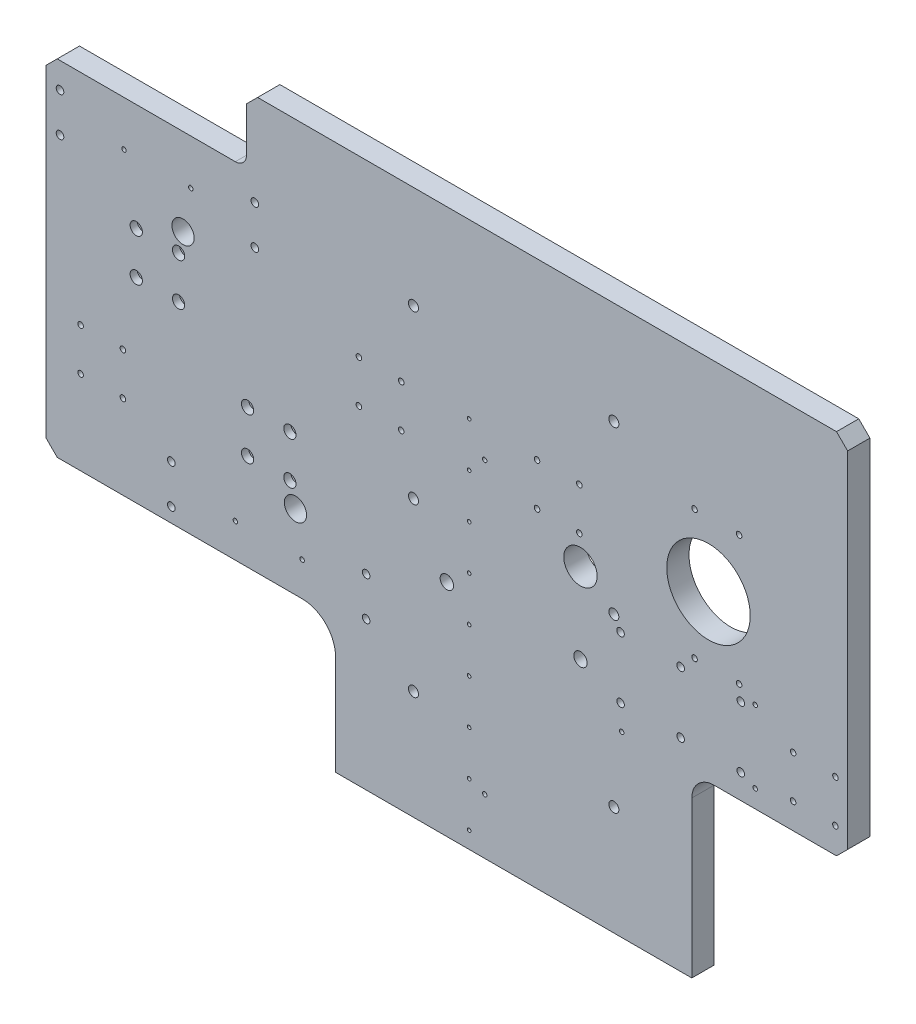
from build123d import *

# Parameters (mm, degrees)
BOSS_EXTRUDE3_DEPTH                                  = 20
CHAMFER1_SIZE                                        = 10
CUT_EXTRUDE3_DEPTH                                   = 697.867993238
CHAMFER2_SIZE                                        = 10
SKETCH20_R                                           = 15
CUT_EXTRUDE5_DEPTH                                   = 697.867993238
M6_TAPPED_HOLE1_D                                    = 5
M8_TAPPED_HOLE1_D                                    = 6.8
M4_TAPPED_HOLE1_D                                    = 3.3
SKETCH30_R                                           = 37.5
CUT_EXTRUDE6_DEPTH                                   = 697.867993238
HOLE_SIZE_PER_SOCKET_HEAD_CAP_SCREW_TYPE_D           = 9
HOLE_SIZE_PER_SOCKET_HEAD_CAP_SCREW_TYPE_CBORE_D     = 15
HOLE_SIZE_PER_SOCKET_HEAD_CAP_SCREW_TYPE_CBORE_DEPTH = 9
SKETCH34_R                                           = 6
CUT_EXTRUDE7_DEPTH                                   = 697.867993238
M6_TAPPED_HOLE2_D                                    = 5
SKETCH37_W                                           = 180
SKETCH37_H                                           = 60
CUT_EXTRUDE8_DEPTH                                   = 697.867993238
LPATTERN1_COUNT                                      = 9
LPATTERN1_PITCH                                      = 40
CBORE_FOR_M6_HEX_SOCKET_HEAD_CAP_SCREW1_D            = 6.6
CBORE_FOR_M6_HEX_SOCKET_HEAD_CAP_SCREW1_CBORE_D      = 11
CBORE_FOR_M6_HEX_SOCKET_HEAD_CAP_SCREW1_CBORE_DEPTH  = 6.4
CHAMFER3_SIZE                                        = 10
FILLET1_R                                            = 10
SKETCH40_R                                           = 10
CUT_EXTRUDE9_DEPTH                                   = 697.867993238
M8_TAPPED_HOLE2_D                                    = 6.8
M8_TAPPED_HOLE2_DEPTH                                = 22.25
M8_TAPPED_HOLE2_TIP                                  = 2.042926105
SKETCH43_R                                           = 2
CUT_EXTRUDE10_DEPTH                                  = 697.867993238
SKETCH44_R                                           = 2
CUT_EXTRUDE11_DEPTH                                  = 697.867993238
SKETCH45_R                                           = 2
CUT_EXTRUDE12_DEPTH                                  = 697.867993238
M6_TAPPED_HOLE3_D                                    = 5
M6_TAPPED_HOLE3_DEPTH                                = 15
M6_TAPPED_HOLE3_TIP                                  = 1.502151548


with BuildPart() as part:
    # Sketch2 → Boss-Extrude3 (new body)
    with BuildSketch(Plane.XY):
        with BuildLine():
            Line((-144.12756851, -271.913182542), (85.87243149, -271.913182542))
            ThreePointArc((85.87243149, -271.913182542), (107.085634925, -280.699979106), (115.87243149, -301.913182542))
            Line((115.87243149, -301.913182542), (115.87243149, -391.913182542))
            Line((115.87243149, -391.913182542), (575.87243149, -391.913182542))
            Line((575.87243149, -391.913182542), (575.87243149, 98.086817458))
            Line((575.87243149, 98.086817458), (-144.12756851, 98.086817458))
            Line((-144.12756851, 98.086817458), (-144.12756851, -271.913182542))
        make_face()
    extrude(amount=BOSS_EXTRUDE3_DEPTH)

    # Chamfer1
    chamfer1_edges = [part.edges().sort_by_distance(p)[0] for p in [
        (-144.12756851, -271.913182542, 10),
        (-144.12756851, 98.086817458, 10),
        (575.87243149, 98.086817458, 10),
    ]]
    chamfer(chamfer1_edges, length=CHAMFER1_SIZE)

    # Sketch6 → Cut-Extrude3 (cut, through all)
    with BuildSketch(Plane(origin=(0, 0, 0), x_dir=(-1, 0, 0), z_dir=(0, 0, -1))):
        with BuildLine():
            Line((-575.87243149, -391.913182542), (-435.87243149, -391.913182542))
            Line((-435.87243149, -391.913182542), (-435.87243149, -251.913182542))
            ThreePointArc((-435.87243149, -251.913182542), (-441.730295866, -237.771046918), (-455.87243149, -231.913182542))
            Line((-455.87243149, -231.913182542), (-575.87243149, -231.913182542))
            Line((-575.87243149, -231.913182542), (-575.87243149, -391.913182542))
        make_face()
    extrude(amount=-CUT_EXTRUDE3_DEPTH, mode=Mode.SUBTRACT)

    # Chamfer2
    chamfer2_edges = [part.edges().sort_by_distance(p)[0] for p in [
        (575.87243149, -231.913182542, 10),
    ]]
    chamfer(chamfer2_edges, length=CHAMFER2_SIZE)

    # Sketch20 → Cut-Extrude5 (cut, through all)
    with BuildSketch(Plane(origin=(0, 0, 0), x_dir=(-1, 0, 0), z_dir=(0, 0, -1))):
        with Locations((-335.87243149, -121.913182542)):
            Circle(SKETCH20_R)
    extrude(amount=-CUT_EXTRUDE5_DEPTH, mode=Mode.SUBTRACT)

    # M6 Tapped Hole1 (through all)
    with Locations(Plane.XY.offset(20)):
        with Locations((438.37243149, -25.913182542), (478.37243149, -25.913182542), (478.37243149, -141.913182542), (438.37243149, -141.913182542)):
            Hole(M6_TAPPED_HOLE1_D / 2)

    # M8 Tapped Hole1 (through all)
    with Locations(Plane(origin=(0, 0, 0), x_dir=(-1, 0, 0), z_dir=(0, 0, -1))):
        with Locations((-425.87243149, -209.913182542), (-425.87243149, -154.913182542), (-371.87243149, -154.913182542), (-371.87243149, -209.913182542), (-479.87243149, -154.913182542), (-479.87243149, -209.913182542)):
            Hole(M8_TAPPED_HOLE1_D / 2)

    # M4 Tapped Hole1 (through all)
    with Locations(Plane(origin=(0, 0, 0), x_dir=(-1, 0, 0), z_dir=(0, 0, -1))):
        with Locations((-235.87243149, -376.913182542)):
            m4_tapped_hole1 = Hole(M4_TAPPED_HOLE1_D / 2)

    # Sketch30 → Cut-Extrude6 (cut, through all)
    with BuildSketch(Plane.XY.offset(20)):
        with Locations((450.87243149, -83.913182542)):
            Circle(SKETCH30_R)
    extrude(amount=-CUT_EXTRUDE6_DEPTH, mode=Mode.SUBTRACT)

    # Hole size per socket head cap screw type 1 (through all)
    with Locations(Plane(origin=(0, 0, 0), x_dir=(-1, 0, 0), z_dir=(0, 0, -1))):
        with Locations((-185.87243149, 6.086817458), (-365.87243149, 6.086817458), (-365.87243149, -143.913182542), (-185.87243149, -143.913182542), (-365.87243149, -293.913182542), (-185.87243149, -293.913182542)):
            CounterBoreHole(HOLE_SIZE_PER_SOCKET_HEAD_CAP_SCREW_TYPE_D / 2, HOLE_SIZE_PER_SOCKET_HEAD_CAP_SCREW_TYPE_CBORE_D / 2, HOLE_SIZE_PER_SOCKET_HEAD_CAP_SCREW_TYPE_CBORE_DEPTH)

    # Sketch34 → Cut-Extrude7 (cut, through all)
    with BuildSketch(Plane(origin=(0, 0, 0), x_dir=(-1, 0, 0), z_dir=(0, 0, -1))):
        with Locations((-335.87243149, -193.913182542)):
            Circle(SKETCH34_R)
        with Locations((-215.87243149, -193.913182542)):
            Circle(SKETCH34_R)
    extrude(amount=-CUT_EXTRUDE7_DEPTH, mode=Mode.SUBTRACT)

    # M6 Tapped Hole2 (through all)
    with Locations(Plane(origin=(0, 0, 0), x_dir=(-1, 0, 0), z_dir=(0, 0, -1))):
        with Locations((-564.87243149, -170.913182542), (-526.87243149, -170.913182542), (-526.87243149, -208.913182542), (-564.87243149, -208.913182542), (-334.87243149, -58.413182542), (-296.87243149, -58.413182542), (-296.87243149, -96.413182542), (-334.87243149, -96.413182542), (-174.87243149, -58.413182542), (-136.87243149, -58.413182542), (-136.87243149, -96.413182542), (-174.87243149, -96.413182542), (75.12756851, -158.413182542), (113.12756851, -158.413182542), (113.12756851, -196.413182542), (75.12756851, -196.413182542)):
            Hole(M6_TAPPED_HOLE2_D / 2)

    # Sketch37 → Cut-Extrude8 (cut, through all)
    with BuildSketch(Plane(origin=(0, 0, 0), x_dir=(-1, 0, 0), z_dir=(0, 0, -1))):
        with Locations((54.12756851, 68.086817458)):
            Rectangle(SKETCH37_W, SKETCH37_H)
    extrude(amount=-CUT_EXTRUDE8_DEPTH, mode=Mode.SUBTRACT)

    # LPattern1: M4 Tapped Hole1 ×9
    with Locations(*[(0, i * LPATTERN1_PITCH, 0) for i in range(1, LPATTERN1_COUNT)]):
        add(m4_tapped_hole1, mode=Mode.SUBTRACT)

    # CBORE for M6 Hex Socket Head Cap Screw1 (through all)
    with Locations(Plane.XY.offset(20)):
        with Locations((36.87243149, -147.413182542), (74.87243149, -147.413182542), (74.87243149, -185.413182542), (36.87243149, -185.413182542), (-25.12756851, -58.413182542), (-63.12756851, -58.413182542), (-63.12756851, -96.413182542), (-25.12756851, -96.413182542)):
            CounterBoreHole(CBORE_FOR_M6_HEX_SOCKET_HEAD_CAP_SCREW1_D / 2, CBORE_FOR_M6_HEX_SOCKET_HEAD_CAP_SCREW1_CBORE_D / 2, CBORE_FOR_M6_HEX_SOCKET_HEAD_CAP_SCREW1_CBORE_DEPTH)

    # Chamfer3
    chamfer3_edges = [part.edges().sort_by_distance(p)[0] for p in [
        (35.87243149, 98.086817458, 10),
        (-144.12756851, 38.086817458, 10),
    ]]
    chamfer(chamfer3_edges, length=CHAMFER3_SIZE)

    # Fillet1
    fillet1_edges = [part.edges().sort_by_distance(p)[0] for p in [
        (35.87243149, 38.086817458, 10),
    ]]
    fillet(fillet1_edges, radius=FILLET1_R)

    # Sketch40 → Cut-Extrude9 (cut, through all)
    with BuildSketch(Plane.XY.offset(20)):
        with Locations((79.87243149, -204.913182542)):
            Circle(SKETCH40_R)
        with Locations((-21.12756851, -39.913182542)):
            Circle(SKETCH40_R)
    extrude(amount=-CUT_EXTRUDE9_DEPTH, mode=Mode.SUBTRACT)

    # M8 Tapped Hole2
    with Locations(Plane(origin=(0, 0, 0), x_dir=(-1, 0, 0), z_dir=(0, 0, -1))):
        with Locations((-43.37243149, 15.086817458), (-43.37243149, -19.913182542), (131.62756851, 15.086817458), (-143.37243149, -223.913182542), (-143.37243149, -258.913182542), (31.62756851, -223.913182542), (31.62756851, -258.913182542), (131.62756851, -19.913182542)):
            Hole(M8_TAPPED_HOLE2_D / 2, depth=M8_TAPPED_HOLE2_DEPTH)
            with Locations((0, 0, -(M8_TAPPED_HOLE2_DEPTH + M8_TAPPED_HOLE2_TIP / 2))):  # 118° drill point
                Cone(0, M8_TAPPED_HOLE2_D / 2, M8_TAPPED_HOLE2_TIP, mode=Mode.SUBTRACT)

    # Sketch43 → Cut-Extrude10 (cut, through all)
    with BuildSketch(Plane(origin=(0, 0, 0), x_dir=(-1, 0, 0), z_dir=(0, 0, -1))):
        with Locations((14.12756851, -2.413182542)):
            Circle(SKETCH43_R)
        with Locations((74.12756851, -2.413182542)):
            Circle(SKETCH43_R)
        with Locations((-85.87243149, -241.413182542)):
            Circle(SKETCH43_R)
        with Locations((-25.87243149, -241.413182542)):
            Circle(SKETCH43_R)
    extrude(amount=-CUT_EXTRUDE10_DEPTH, mode=Mode.SUBTRACT)

    # Sketch44 → Cut-Extrude11 (cut, through all)
    with BuildSketch(Plane(origin=(0, 0, 0), x_dir=(-1, 0, 0), z_dir=(0, 0, -1))):
        with Locations((-249.87243149, -341.913182542)):
            Circle(SKETCH44_R)
        with Locations((-249.87243149, -81.913182542)):
            Circle(SKETCH44_R)
    extrude(amount=-CUT_EXTRUDE11_DEPTH, mode=Mode.SUBTRACT)

    # Sketch45 → Cut-Extrude12 (cut, through all)
    with BuildSketch(Plane(origin=(0, 0, 0), x_dir=(-1, 0, 0), z_dir=(0, 0, -1))):
        with Locations((-492.87243149, -150.913182542)):
            Circle(SKETCH45_R)
        with Locations((-492.87243149, -215.913182542)):
            Circle(SKETCH45_R)
        with Locations((-372.87243149, -231.913182542)):
            Circle(SKETCH45_R)
    extrude(amount=-CUT_EXTRUDE12_DEPTH, mode=Mode.SUBTRACT)

    # M6 Tapped Hole3
    with Locations(Plane(origin=(0, 0, 0), x_dir=(-1, 0, 0), z_dir=(0, 0, -1))):
        with Locations((112.27756851, -118.513182542), (132.12756851, -116.913182542)):
            Hole(M6_TAPPED_HOLE3_D / 2, depth=M6_TAPPED_HOLE3_DEPTH)
            with Locations((0, 0, -(M6_TAPPED_HOLE3_DEPTH + M6_TAPPED_HOLE3_TIP / 2))):  # 118° drill point
                Cone(0, M6_TAPPED_HOLE3_D / 2, M6_TAPPED_HOLE3_TIP, mode=Mode.SUBTRACT)


solid = part.part
